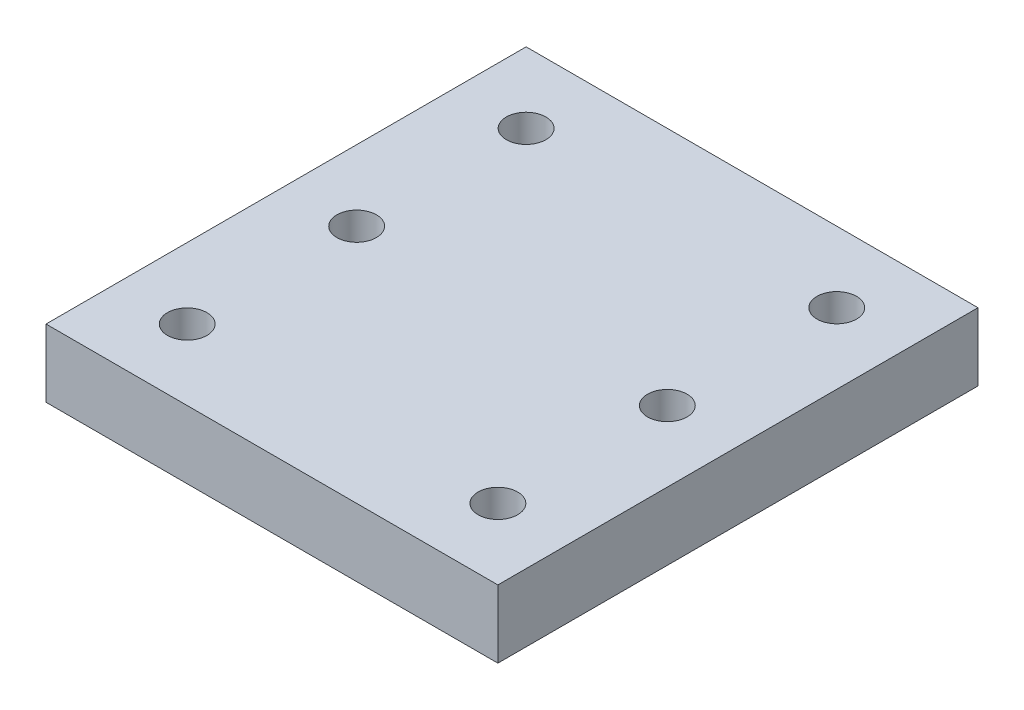
from build123d import *

# Parameters (mm, degrees)
SKETCH_1_W          = 160
SKETCH_1_H          = 170
EXTRUDE_1_DEPTH     = 24
HOLE_WIZARD_M16_1_D = 14


with BuildPart() as part:
    # 草图1 → 凸台-拉伸1 (new body)
    with BuildSketch(Plane(origin=(0, 0, 0), x_dir=(1, 0, 0), z_dir=(0, 1, 0))):
        Rectangle(SKETCH_1_W, SKETCH_1_H)
    extrude(amount=EXTRUDE_1_DEPTH)

    # M16 螺纹孔1 (through all)
    with Locations(Plane(origin=(0, 24, 0), x_dir=(1, 0, 0), z_dir=(0, 1, 0))):
        with Locations((-55, -60), (-55, 60), (55, 60), (55, -60), (55, 0), (-55, 0)):
            Hole(HOLE_WIZARD_M16_1_D / 2)


solid = part.part
